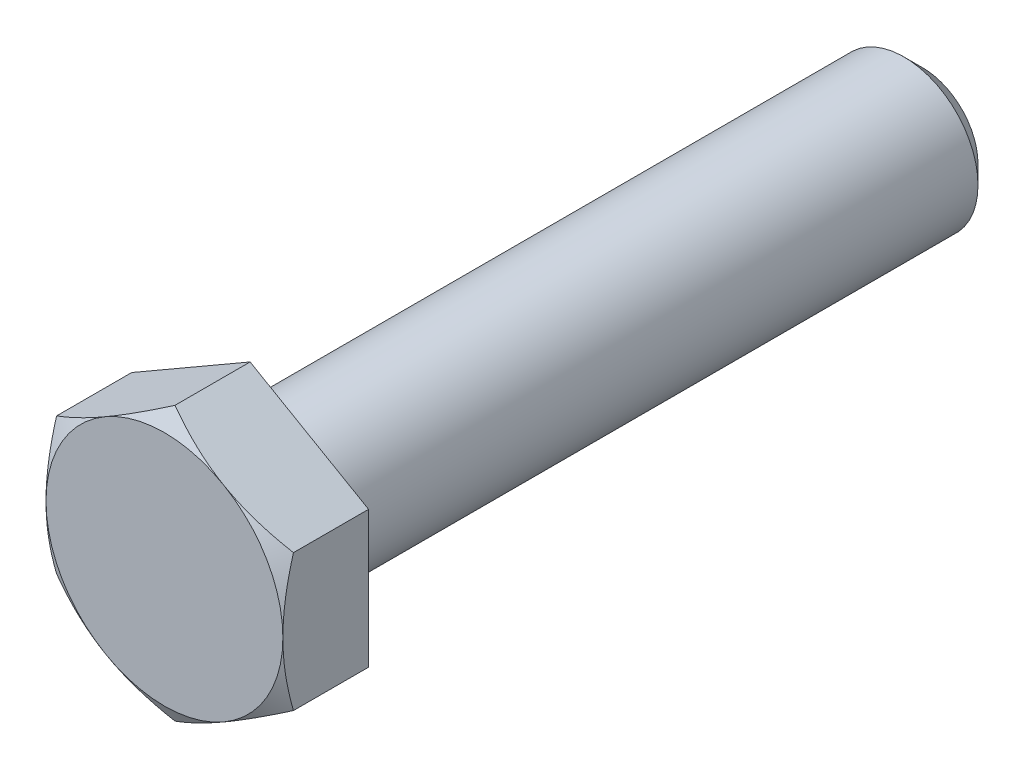
from build123d import *

# Parameters (mm, degrees)
EXTRUDE_1_DEPTH     = 6.2
SKETCH_3_R          = 5
EXTRUDE_3_DEPTH     = 45
SKETCH_5_OUTSIDE_W  = 375.758
SKETCH_5_OUTSIDE_H  = 378.234
SKETCH_5_OUTSIDE_R  = 8
CUT_EXTRUDE_2_DEPTH = 100
CUT_EXTRUDE_2_DRAFT = -60
CHAMFER_1_SIZE      = 1.25
SKETCH_2_OUTSIDE_W  = 29.346
SKETCH_2_OUTSIDE_H  = 31.822
SKETCH_2_OUTSIDE_R  = 7.2
CUT_EXTRUDE_1_DEPTH = 0.413333333
FILLET_1_R          = 0.1


with BuildPart() as part:
    # 草图1 → 凸台-拉伸1 (new body)
    with BuildSketch(Plane.XY):
        Polygon((0, 9.237604307), (-8, 4.618802154), (-8, -4.618802154), (0, -9.237604307), (8, -4.618802154), (8, 4.618802154), align=None)
    extrude(amount=EXTRUDE_1_DEPTH)

    # 草图3 → 凸台-拉伸3 (add)
    with BuildSketch(Plane.XY):
        Circle(SKETCH_3_R)
    extrude(amount=-EXTRUDE_3_DEPTH)


with BuildPart() as cut_extrude_2_tool:
    # 草图5 outside → 切除-拉伸2 (with draft: the straight prism first)
    with BuildSketch(Plane.XY.offset(6.2)):
        Rectangle(SKETCH_5_OUTSIDE_W, SKETCH_5_OUTSIDE_H)
        Circle(SKETCH_5_OUTSIDE_R, mode=Mode.SUBTRACT)
    extrude(amount=-CUT_EXTRUDE_2_DEPTH)
    # 切除-拉伸2: the draft: its side faces are tilted about the plane it starts from
    cut_extrude_2_sides = [cut_extrude_2_tool.faces().sort_by_distance(p)[0] for p in [
        (0, -189.117, -43.8),
        (187.879, 0, -43.8),
        (0, 189.117, -43.8),
        (-187.879, 0, -43.8),
        (-8, 0, -43.8),
    ]]
    draft(cut_extrude_2_sides, Plane.XY.offset(6.2), CUT_EXTRUDE_2_DRAFT)


with BuildPart() as part_1:
    add(part.part)

    # 切除-拉伸2: cut by cut_extrude_2_tool
    add(cut_extrude_2_tool.part, mode=Mode.SUBTRACT)

    # 倒角1
    chamfer_1_edges = [part_1.edges().sort_by_distance(p)[0] for p in [
        (-5, 0, -45),
    ]]
    chamfer(chamfer_1_edges, length=CHAMFER_1_SIZE)

    # 草图2 outside → 切除-拉伸1 (cut)
    with BuildSketch(Plane.XY):
        Rectangle(SKETCH_2_OUTSIDE_W, SKETCH_2_OUTSIDE_H)
        Circle(SKETCH_2_OUTSIDE_R, mode=Mode.SUBTRACT)
    extrude(amount=CUT_EXTRUDE_1_DEPTH, mode=Mode.SUBTRACT)

    # 圆角1
    fillet_1_edges = [part_1.edges().sort_by_distance(p)[0] for p in [
        (-5, 0, 0),
    ]]
    fillet(fillet_1_edges, radius=FILLET_1_R)


solid = part_1.part
